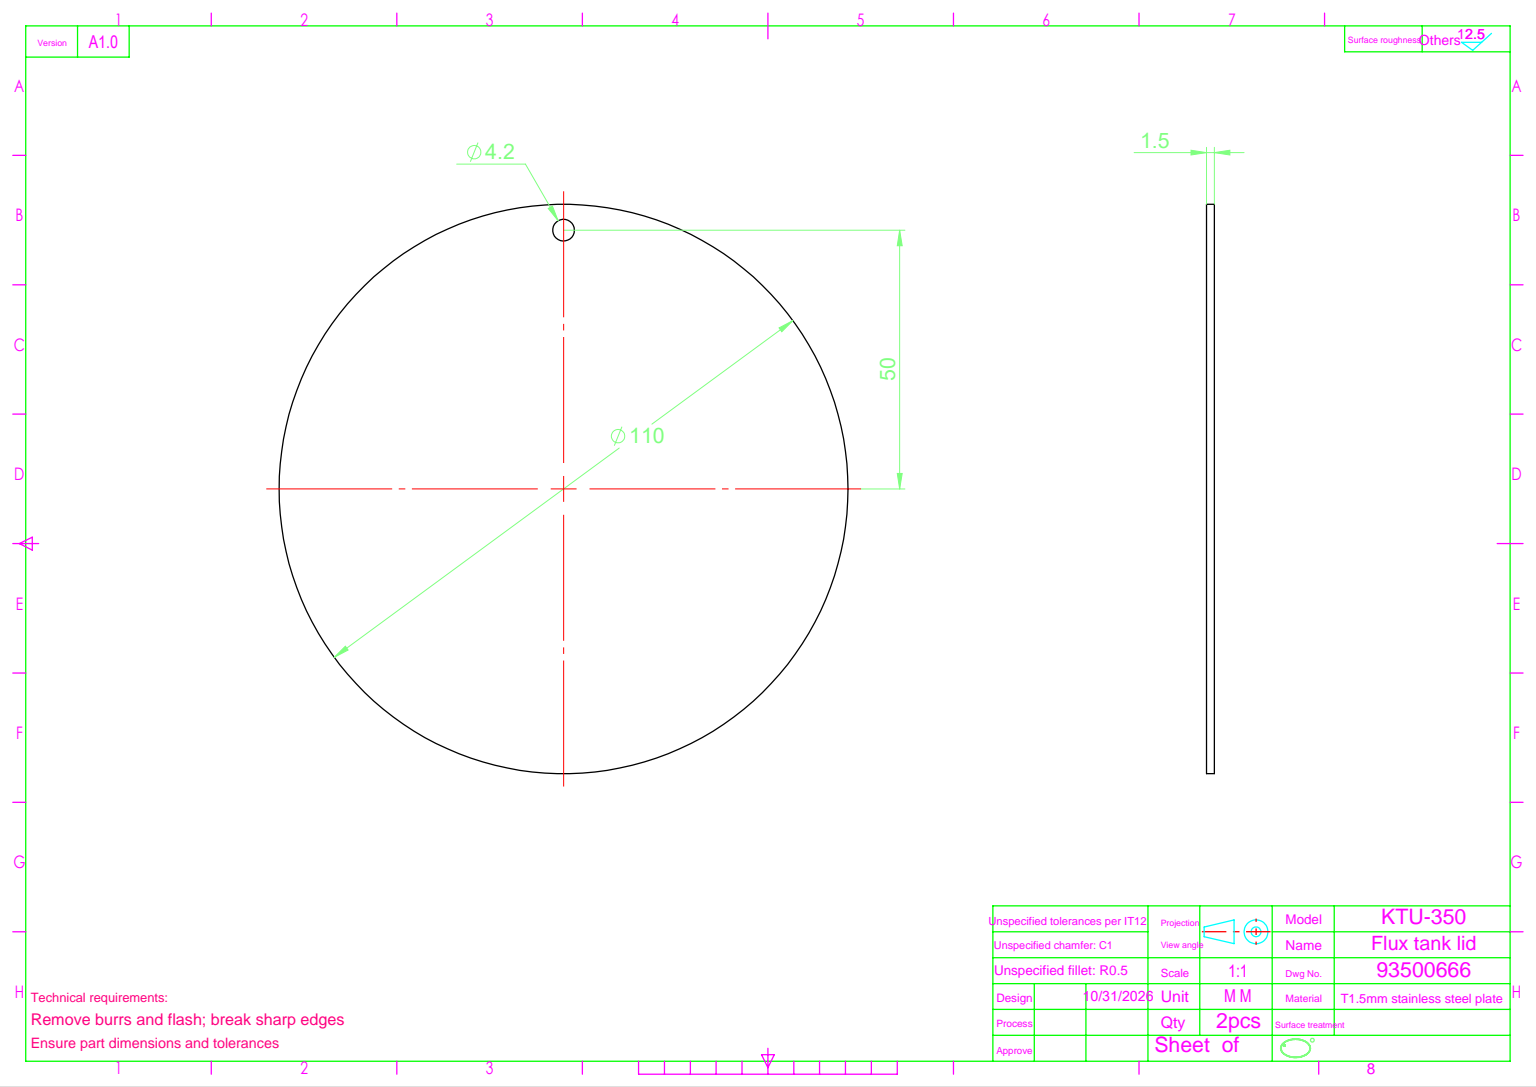
SolidWorks part; units mm, degrees
ref_plane "前视" through (0, 0, 0) normal (0, 0, 1) x (1, 0, 0)
ref_plane "上视" through (0, 0, 0) normal (0, 1, 0) x (1, 0, 0)
ref_plane "右视" through (0, 0, 0) normal (1, 0, 0) x (0, 0, -1)
sketch "草图1" plane through (0, 0, 0) normal (0, 0, 1) x (1, 0, 0)
  circle A0 centre (0, 0) radius 55
  dimension "D1" = 110
extrude "凸台-拉伸1" add sketch "草图1" along normal blind 1.5
sketch "草图2" plane through (0, 0, 1.5) normal (0, 0, 1) x (1, 0, 0)
  circle A0 centre (0, 50) radius 2.1
  dimension "D1" = 4.2
  dimension "D2" = 50
extrude "切除-拉伸1" cut sketch "草图2" against normal blind 1.5
